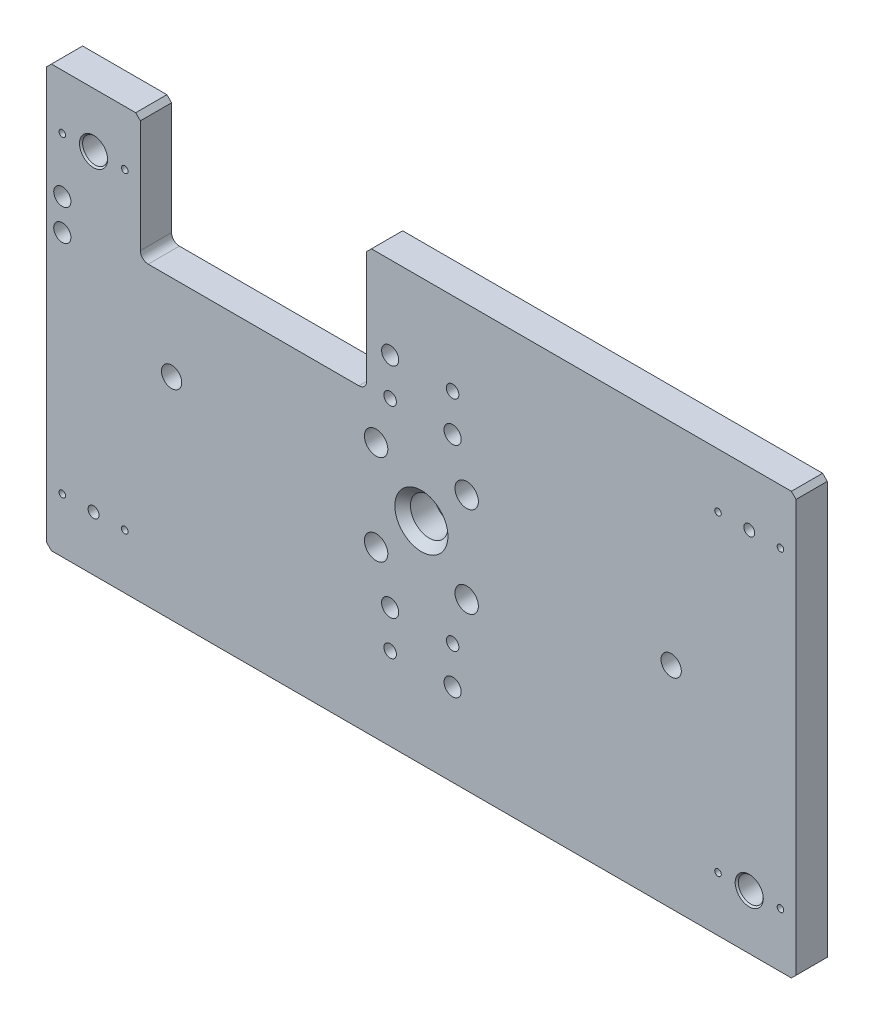
SolidWorks part; units mm, degrees
material "Q235-A"
ref_plane "Front Plane" through (0, 0, 0) normal (0, 0, 1) x (1, 0, 0)
ref_plane "Top Plane" through (0, 0, 0) normal (0, 1, 0) x (1, 0, 0)
ref_plane "Right Plane" through (0, 0, 0) normal (1, 0, 0) x (0, 0, -1)
sketch "Sketch1" plane through (0, 0, 0) normal (0, 0, 1) x (1, 0, 0)
  line L0 (18.0373, 176.5929) -> (293.0373, 176.5929)
  line L1 (-186.9627, 176.5929) -> (-126.9627, 176.5929)
  line L2 (-186.9627, 176.5929) -> (-186.9627, -93.4071)
  line L3 (-186.9627, -93.4071) -> (293.0373, -93.4071)
  line L4 (293.0373, 176.5929) -> (293.0373, -93.4071)
  line L6 (-126.9627, 176.5929) -> (-126.9627, 96.5929)
  line L7 (-126.9627, 96.5929) -> (18.0373, 96.5929)
  line L8 (18.0373, 176.5929) -> (18.0373, 96.5929)
  dimension "D1" = 480
  dimension "D2" = 270
  dimension "D3" = 80
  dimension "D4" = 145
  dimension "D5" = 60
extrude "Boss-Extrude1" add sketch "Sketch1" along normal blind 20
sketch "Sketch3" plane through (0, 0, 20) normal (0, 0, 1) x (1, 0, 0)
  line L0 (-156.9627, 141.5929) -> (263.0373, 141.5929)
  line L1 (-156.9627, 141.5929) -> (-156.9627, -58.4071)
  line L2 (-156.9627, -58.4071) -> (263.0373, -58.4071)
  line L3 (263.0373, 141.5929) -> (263.0373, -58.4071)
  line L4 (-186.9627, -93.4071) -> (293.0373, -93.4071) construction
  line L5 (-186.9627, 176.5929) -> (-186.9627, -93.4071) construction
  line L6 (-176.9627, 106.5929) -> (-176.9627, 86.5929)
  line L7 (-106.9627, 41.5929) -> (213.0373, 41.5929)
  line L9 (24.0373, 12.5929) -> (82.0373, 12.5929)
  line L10 (24.0373, 12.5929) -> (24.0373, 70.5929)
  line L11 (24.0373, 70.5929) -> (82.0373, 70.5929)
  line L12 (82.0373, 12.5929) -> (82.0373, 70.5929)
  line L13 (24.0373, 12.5929) -> (82.0373, 70.5929) construction
  line L14 (24.0373, 70.5929) -> (82.0373, 12.5929) construction
  line L15 (33.0373, 123.5929) -> (73.0373, 123.5929)
  line L16 (33.0373, 123.5929) -> (33.0373, 99.5929)
  line L17 (33.0373, 99.5929) -> (73.0373, 99.5929)
  line L18 (73.0373, 123.5929) -> (73.0373, 99.5929)
  line L19 (33.0373, -16.4071) -> (73.0373, -16.4071)
  line L20 (33.0373, -16.4071) -> (33.0373, -40.4071)
  line L21 (33.0373, -40.4071) -> (73.0373, -40.4071)
  line L22 (73.0373, -16.4071) -> (73.0373, -40.4071)
  circle A0 centre (-136.9627, -58.4071) radius 6.7804
  circle A1 centre (-176.9627, -58.4071) radius 5.9501
  circle A2 centre (-136.9627, 141.5929) radius 6.7804
  circle A4 centre (283.0373, 141.5929) radius 6.7804
  circle A5 centre (243.0373, 141.5929) radius 5.9501
  circle A6 centre (283.0373, -58.4071) radius 6.7804
  circle A7 centre (243.0373, -58.4071) radius 5.9501
  circle A8 centre (-136.9627, -58.4071) radius 6.7804
  circle A9 centre (-176.9627, -58.4071) radius 5.9501
  circle A10 centre (53.0373, 41.5929) radius 14.1494
  circle A11 centre (-176.9627, 141.5929) radius 6.7273
  dimension "D6" = 20
  dimension "D1" = 420
  dimension "D2" = 200
  dimension "D3" = 35
  dimension "D4" = 30
  dimension "D5" = 20
  dimension "D7" = 20
  dimension "D8" = 180
  dimension "D9" = 320
  dimension "D10" = 80
  dimension "D11" = 100
  dimension "D12" = 58
  dimension "D13" = 58
  dimension "D14" = 40
  dimension "D15" = 24
  dimension "D16" = 58
  dimension "D17" = 40
  dimension "D18" = 24
  dimension "D19" = 58
  dimension "D20" = 20
  dimension "D21" = 20
fillet "Fillet1" radius 5 2 edges at (18.0373, 96.5929, 10) (-126.9627, 96.5929, 10)
chamfer "Chamfer1" distance 3 angle 45 6 edges at (-186.9627, -93.4071, 10) (293.0373, -93.4071, 10) (293.0373, 176.5929, 10) (18.0373, 176.5929, 10) (-126.9627, 176.5929, 10) (-186.9627, 176.5929, 10)
hole_wizard "Hole2" positions "Sketch4" profile "Sketch5" legacy end condition through all
sketch "Sketch4" plane through (0, 0, 20) normal (0, 0, 1) x (1, 0, 0)
  point P0 (-176.9627, 106.5929)
  point P3 (-176.9627, 86.5929)
sketch "Sketch5" plane through (-176.9627, 106.5929, 20) normal (1, 0, 0) x (0, -1, 0)
  line L0 (0, 0) -> (0, 20)
  line L1 (0, 20) -> (3.3, 20)
  line L2 (3.3, 20) -> (3.3, 9)
  line L3 (3.3, 9) -> (5.5, 9)
  line L4 (5.5, 9) -> (5.5, 0)
  line L5 (5.5, 0) -> (0, 0)
  line L6 (0, 110) -> (0, -10) construction
  dimension "直径" = 6.6
  dimension "深度" = 20
  dimension "柱坑直径" = 11
  dimension "柱坑深度" = 9
hole_wizard "M5 Tapped Hole1" positions "Sketch6" profile "Sketch7" tap size "M5" standard "GB"
sketch "Sketch6" plane through (0, 0, 20) normal (0, 0, 1) x (1, 0, 0)
  point P0 (-176.9627, 141.5929)
  point P3 (-136.9627, 141.5929)
  point P6 (-176.9627, -58.4071)
  point P9 (-136.9627, -58.4071)
  point P12 (243.0373, -58.4071)
  point P15 (283.0373, -58.4071)
  point P18 (283.0373, 141.5929)
  point P21 (243.0373, 141.5929)
sketch "Sketch7" plane through (-176.9627, 141.5929, 20) normal (1, 0, 0) x (0, -1, 0)
  line L0 (0, 0) -> (0, 11.2618)
  line L1 (0, 11.2618) -> (2.1, 10)
  line L2 (2.1, 10) -> (2.1, 0)
  line L5 (2.1, 0) -> (0, 0)
  line L10 (0, 11.2618) -> (-2.1, 10) construction
  line L11 (0, -6.35) -> (0, 107.95) construction
  dimension "螺纹孔钻头直径" = 4.2
  dimension "螺纹孔钻头深度" = 10
  dimension "导头角度" = 118
cosmetic thread "Cosmetic thread 1" parameters "D1"=10, "D2"=5
cosmetic thread "Cosmetic thread 2" parameters "D1"=10, "D2"=5
cosmetic thread "Cosmetic thread 3" parameters "D1"=10, "D2"=5
cosmetic thread "Cosmetic thread 4" parameters "D1"=10, "D2"=5
cosmetic thread "Cosmetic thread 5" parameters "D1"=10, "D2"=5
cosmetic thread "Cosmetic thread 6" parameters "D1"=10, "D2"=5
cosmetic thread "Cosmetic thread 7" parameters "D1"=10, "D2"=5
cosmetic thread "Cosmetic thread 8" parameters "D1"=10, "D2"=5
hole_wizard "M8x1.0 Tapped Hole1" positions "Sketch8" profile "Sketch9" tap size "M8x1.0" standard "GB" end condition through all
sketch "Sketch8" plane through (0, 0, 20) normal (0, 0, 1) x (1, 0, 0)
  point P0 (-156.9627, -58.4071)
  point P3 (263.0373, 141.5929)
sketch "Sketch9" plane through (-156.9627, -58.4071, 20) normal (1, 0, 0) x (0, -1, 0)
  line L0 (0, 0) -> (0, 20)
  line L1 (0, 20) -> (3.5, 20)
  line L2 (3.5, 20) -> (3.5, 0)
  line L5 (3.5, 0) -> (0, 0)
  line L11 (0, -6.35) -> (0, 107.95) construction
  dimension "通孔螺纹孔钻头直径" = 7
  dimension "通孔螺纹孔钻头深度" = 20
cosmetic thread "Cosmetic thread 9" parameters "D2"=8
cosmetic thread "Cosmetic thread 10" parameters "D2"=8
hole_wizard "Hole3" positions "Sketch10" profile "Sketch11" legacy end condition through all
sketch "Sketch10" plane through (0, 0, 20) normal (0, 0, 1) x (1, 0, 0)
  point P0 (-156.9627, 141.5929)
  point P3 (263.0373, -58.4071)
sketch "Sketch11" plane through (-156.9627, 141.5929, 20) normal (1, 0, 0) x (0, -1, 0)
  line L0 (0, 0) -> (0, 20)
  line L1 (0, 20) -> (4.5, 20)
  line L2 (4.5, 20) -> (4.5, 12)
  line L3 (4.5, 12) -> (8, 12)
  line L4 (8, 12) -> (8, 0)
  line L5 (8, 0) -> (0, 0)
  line L6 (0, 110) -> (0, -10) construction
  dimension "直径" = 9
  dimension "深度" = 20
  dimension "柱坑直径" = 16
  dimension "柱坑深度" = 12
hole_wizard "Hole4" positions "Sketch12" profile "Sketch13" legacy end condition through all
sketch "Sketch12" plane through (0, 0, 20) normal (0, 0, 1) x (1, 0, 0)
  point P0 (24.0373, 70.5929)
  point P3 (82.0373, 70.5929)
  point P6 (82.0373, 12.5929)
  point P9 (24.0373, 12.5929)
sketch "Sketch13" plane through (24.0373, 70.5929, 20) normal (1, 0, 0) x (0, -1, 0)
  line L0 (0, 0) -> (0, 20)
  line L1 (0, 20) -> (4.5, 20)
  line L2 (4.5, 20) -> (4.5, 11)
  line L3 (4.5, 11) -> (7.5, 11)
  line L4 (7.5, 11) -> (7.5, 0)
  line L5 (7.5, 0) -> (0, 0)
  line L6 (0, 110) -> (0, -10) construction
  dimension "直径" = 9
  dimension "深度" = 20
  dimension "柱坑直径" = 15
  dimension "柱坑深度" = 11
hole_wizard "Hole5" positions "Sketch14" profile "Sketch15" legacy end condition through all
sketch "Sketch14" plane through (0, 0, 20) normal (0, 0, 1) x (1, 0, 0)
  point P0 (33.0373, 123.5929)
  point P3 (73.0373, 99.5929)
  point P6 (33.0373, -16.4071)
  point P9 (73.0373, -40.4071)
sketch "Sketch15" plane through (33.0373, 123.5929, 20) normal (1, 0, 0) x (0, -1, 0)
  line L0 (0, 0) -> (0, 20)
  line L1 (0, 20) -> (3.3, 20)
  line L2 (3.3, 20) -> (3.3, 9)
  line L3 (3.3, 9) -> (5.5, 9)
  line L4 (5.5, 9) -> (5.5, 0)
  line L5 (5.5, 0) -> (0, 0)
  line L6 (0, 110) -> (0, -10) construction
  dimension "直径" = 6.6
  dimension "深度" = 20
  dimension "柱坑直径" = 11
  dimension "柱坑深度" = 9
hole_wizard "Hole6" positions "Sketch16" profile "Sketch17" legacy end condition through all
sketch "Sketch16" plane through (0, 0, 20) normal (0, 0, 1) x (1, 0, 0)
  point P0 (73.0373, 123.5929)
  point P3 (33.0373, 99.5929)
  point P6 (33.0373, -40.4071)
  point P9 (73.0373, -16.4071)
sketch "Sketch17" plane through (73.0373, 123.5929, 20) normal (1, 0, 0) x (0, -1, 0)
  line L0 (0, 0) -> (0, 20)
  line L1 (0, 20) -> (4, 20)
  line L2 (4, 20) -> (4, 0)
  line L3 (4, 0) -> (0, 0)
  line L4 (0, 110) -> (0, -10) construction
  dimension "直径" = 8
  dimension "深度" = 20
hole_wizard "Hole7" positions "Sketch18" profile "Sketch19" legacy end condition through all
sketch "Sketch18" plane through (0, 0, 20) normal (0, 0, 1) x (1, 0, 0)
  point P0 (53.0373, 41.5929)
sketch "Sketch19" plane through (53.0373, 41.5929, 20) normal (1, 0, 0) x (0, -1, 0)
  line L0 (0, 0) -> (0, 20)
  line L1 (0, 20) -> (12, 20)
  line L2 (12, 20) -> (12, 0)
  line L3 (12, 0) -> (0, 0)
  line L4 (0, 110) -> (0, -10) construction
  dimension "直径" = 24
  dimension "深度" = 20
sketch "Sketch20" plane through (0, 0, 0) normal (0, 0, -1) x (-1, 0, 0)
  line L0 (106.9627, 41.5929) -> (-213.0373, 41.5929) construction
  line L1 (176.9627, 106.5929) -> (176.9627, 86.5929) construction
  line L2 (106.9627, 41.5929) -> (-213.0373, 41.5929)
  line L3 (176.9627, 106.5929) -> (176.9627, 86.5929)
  line L4 (156.9627, 141.5929) -> (-263.0373, 141.5929)
  line L5 (-263.0373, 141.5929) -> (-263.0373, -58.4071)
  line L6 (-263.0373, -58.4071) -> (156.9627, -58.4071)
  line L7 (156.9627, -58.4071) -> (156.9627, 141.5929)
  line L8 (156.9627, 141.5929) -> (-263.0373, 141.5929)
  line L9 (-263.0373, 141.5929) -> (-263.0373, -58.4071)
  line L10 (-263.0373, -58.4071) -> (156.9627, -58.4071)
  line L11 (156.9627, -58.4071) -> (156.9627, 141.5929)
  line L12 (-33.0373, -16.4071) -> (-73.0373, -16.4071)
  line L13 (-73.0373, -16.4071) -> (-73.0373, -40.4071)
  line L14 (-73.0373, -40.4071) -> (-33.0373, -40.4071)
  line L15 (-33.0373, -40.4071) -> (-33.0373, -16.4071)
  line L16 (-33.0373, -16.4071) -> (-73.0373, -16.4071)
  line L17 (-73.0373, -16.4071) -> (-73.0373, -40.4071)
  line L18 (-73.0373, -40.4071) -> (-33.0373, -40.4071)
  line L19 (-33.0373, -40.4071) -> (-33.0373, -16.4071)
  line L20 (-33.0373, 123.5929) -> (-73.0373, 123.5929)
  line L21 (-73.0373, 123.5929) -> (-73.0373, 99.5929)
  line L22 (-73.0373, 99.5929) -> (-33.0373, 99.5929)
  line L23 (-33.0373, 99.5929) -> (-33.0373, 123.5929)
  line L24 (-33.0373, 123.5929) -> (-73.0373, 123.5929)
  line L25 (-73.0373, 123.5929) -> (-73.0373, 99.5929)
  line L26 (-73.0373, 99.5929) -> (-33.0373, 99.5929)
  line L27 (-33.0373, 99.5929) -> (-33.0373, 123.5929)
  line L28 (-82.0373, 12.5929) -> (-24.0373, 12.5929)
  line L29 (-82.0373, 70.5929) -> (-82.0373, 12.5929)
  line L30 (-24.0373, 70.5929) -> (-82.0373, 70.5929)
  line L31 (-24.0373, 12.5929) -> (-24.0373, 70.5929)
  line L32 (-82.0373, 12.5929) -> (-24.0373, 12.5929)
  line L33 (-82.0373, 70.5929) -> (-82.0373, 12.5929)
  line L34 (-24.0373, 70.5929) -> (-82.0373, 70.5929)
  line L35 (-24.0373, 12.5929) -> (-24.0373, 70.5929)
  circle A1 centre (176.9627, 141.5929) radius 6.7273
  circle A2 centre (176.9627, 141.5929) radius 6.7273
  circle A3 centre (136.9627, 141.5929) radius 6.7804
  circle A4 centre (136.9627, 141.5929) radius 6.7804
  circle A5 centre (176.9627, -58.4071) radius 5.9501
  circle A6 centre (176.9627, -58.4071) radius 5.9501
  circle A7 centre (136.9627, -58.4071) radius 6.7804
  circle A8 centre (136.9627, -58.4071) radius 6.7804
  circle A9 centre (176.9627, -58.4071) radius 5.9501
  circle A10 centre (176.9627, -58.4071) radius 5.9501
  circle A11 centre (136.9627, -58.4071) radius 6.7804
  circle A12 centre (136.9627, -58.4071) radius 6.7804
  circle A13 centre (-243.0373, -58.4071) radius 5.9501
  circle A14 centre (-243.0373, -58.4071) radius 5.9501
  circle A15 centre (-283.0373, -58.4071) radius 6.7804
  circle A16 centre (-283.0373, -58.4071) radius 6.7804
  circle A17 centre (-243.0373, 141.5929) radius 5.9501
  circle A18 centre (-243.0373, 141.5929) radius 5.9501
  circle A19 centre (-283.0373, 141.5929) radius 6.7804
  circle A20 centre (-283.0373, 141.5929) radius 6.7804
  circle A21 centre (-53.0373, 41.5929) radius 14.1494
  circle A22 centre (-53.0373, 41.5929) radius 14.1494
  dimension "D1" = 0
  dimension "D2" = 0
  dimension "D3" = 0
  dimension "D4" = 0
  dimension "D5" = 0
  dimension "D6" = 0
  dimension "D7" = 0
  dimension "D8" = 0
  dimension "D9" = 0
  dimension "D10" = 0
  dimension "D11" = 0
  dimension "D12" = 0
  dimension "D13" = 0
  dimension "D14" = 0
  dimension "D15" = 0
hole_wizard "Hole8" positions "Sketch21" profile "Sketch22" legacy end condition through all
sketch "Sketch21" plane through (0, 0, 0) normal (0, 0, -1) x (-1, 0, 0)
  point P0 (-213.0373, 41.5929)
  point P3 (106.9627, 41.5929)
sketch "Sketch22" plane through (213.0373, 41.5929, 0) normal (1, 0, 0) x (0, 1, 0)
  line L0 (0, 0) -> (0, 20)
  line L1 (0, 20) -> (6.5, 20)
  line L2 (6.5, 20) -> (6.5, 8)
  line L3 (6.5, 8) -> (20, 8)
  line L4 (20, 8) -> (20, 0)
  line L5 (20, 0) -> (0, 0)
  line L6 (0, 110) -> (0, -10) construction
  dimension "直径" = 13
  dimension "深度" = 20
  dimension "柱坑直径" = 40
  dimension "柱坑深度" = 8
chamfer "Chamfer2" distance 1 angle 45 4 edges at (-126.9627, 41.5929, 0) (193.0373, 41.5929, 0) (271.0373, -58.4071, 20) (-148.9627, 141.5929, 20)
chamfer "Chamfer3" distance 5 angle 45 1 edges at (65.0373, 41.5929, 20)
